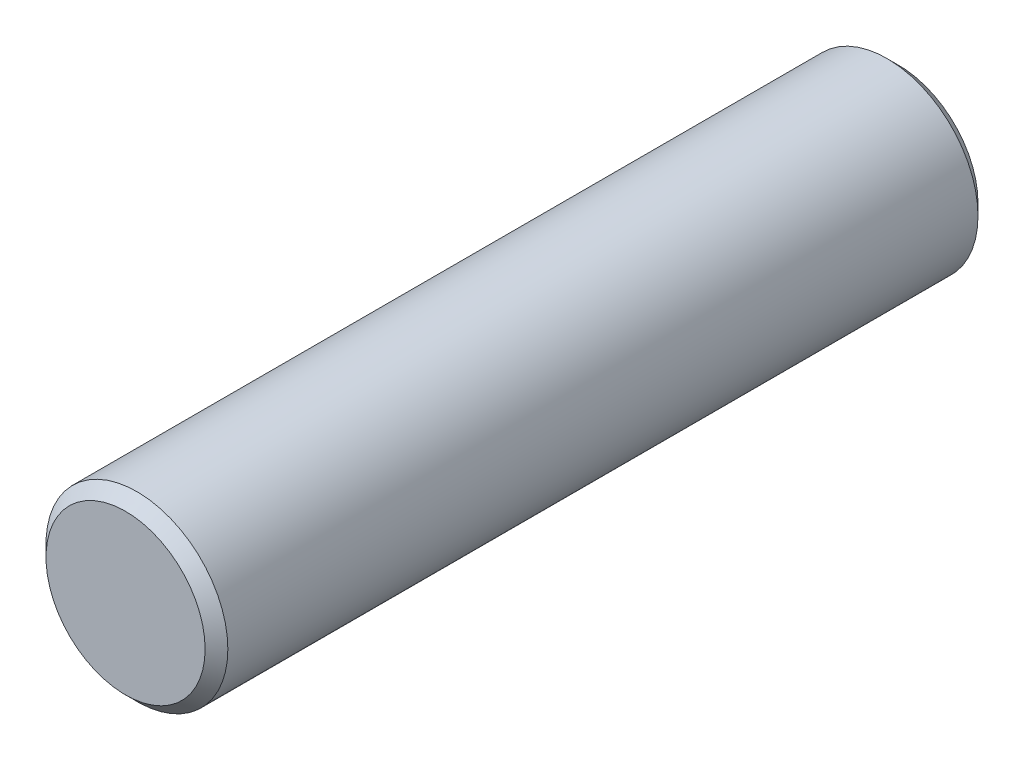
SolidWorks part; units mm, degrees
material "ABS"
ref_plane "Front Plane" through (0, 0, 0) normal (0, 0, 1) x (1, 0, 0)
ref_plane "Top Plane" through (0, 0, 0) normal (0, 1, 0) x (1, 0, 0)
ref_plane "Right Plane" through (0, 0, 0) normal (1, 0, 0) x (0, 0, -1)
sketch "Sketch1" plane through (0, 0, 0) normal (0, 0, 1) x (1, 0, 0)
  circle A0 centre (0, 0) radius 4
  dimension "D1" = 8
extrude "Boss-Extrude1" add sketch "Sketch1" along normal mid plane 34
chamfer "Chamfer1" distance 0.5 angle 45 2 edges at (4, 0, -17) (4, 0, 17)
